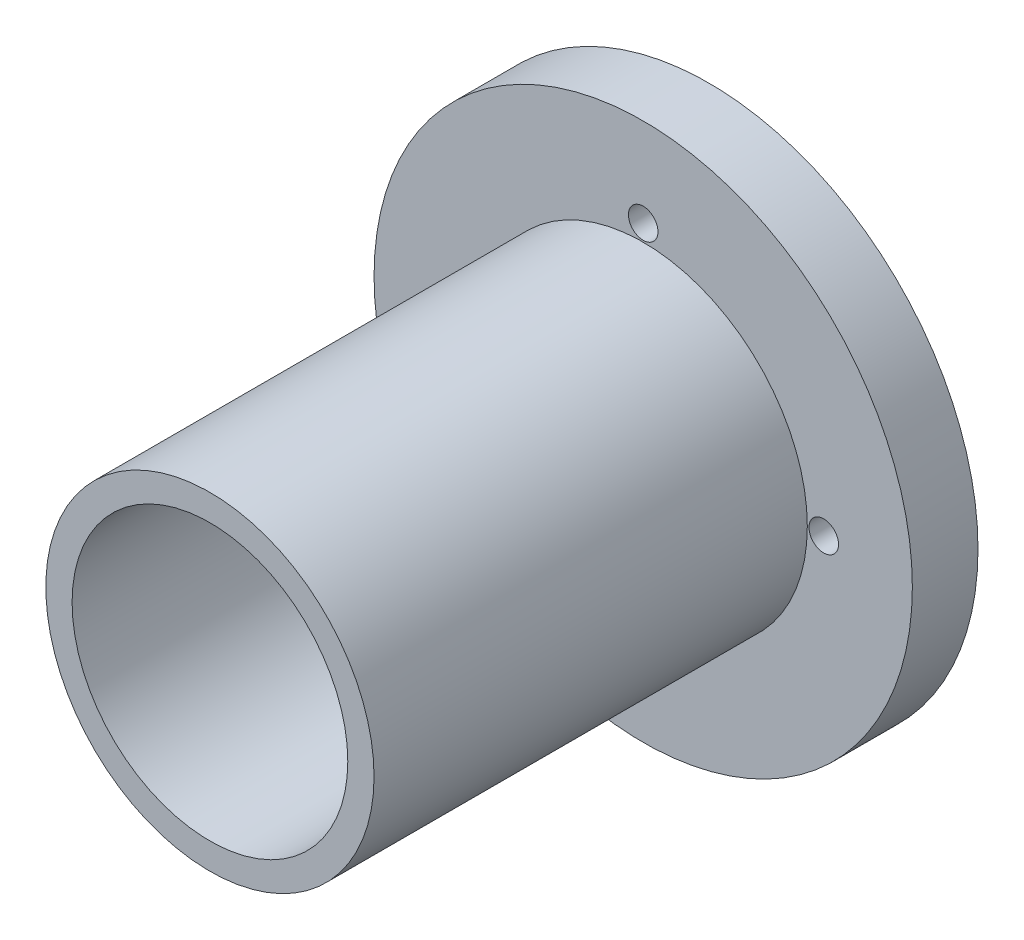
from build123d import *
from build123d.topology import SkipClean

# Parameters (mm, degrees)
SKETCH_1_R                = 25
SKETCH_1_R_2              = 21
EXTRUDE_1_DEPTH           = 66
EXTRUDE_START             = 10
SKETCH_2_R                = 41
SKETCH_2_R_2              = 21
EXTRUDE_2_DEPTH           = 10
HOLE_WIZARD_1_D           = 4.5
HOLE_WIZARD_1_CBORE_D     = 8
HOLE_WIZARD_1_CBORE_DEPTH = 4.6
PATTERN_CIRCULAR_1_COUNT  = 4


with BuildPart() as part:
    # 草图1 → 凸台-拉伸1 (new body)
    with BuildSketch(Plane.XY):
        Circle(SKETCH_1_R)
        Circle(SKETCH_1_R_2, mode=Mode.SUBTRACT)
    extrude(amount=EXTRUDE_1_DEPTH)

    # 草图2 → 凸台-拉伸2 (add)
    with SkipClean():  # the faces are left unmerged after this step: merging them gives an invalid solid
        with BuildSketch(Plane(origin=(0, 0, 0), x_dir=(-1, 0, 0), z_dir=(0, 0, -1)).offset(EXTRUDE_START)):
            Circle(SKETCH_2_R)
            Circle(SKETCH_2_R_2, mode=Mode.SUBTRACT)
        extrude(amount=-EXTRUDE_2_DEPTH)

    # 打孔尺寸(%根据)内六角圆柱头螺钉的类型1 (through all)
    with Locations(Plane(origin=(0, -27.5, -10), x_dir=(-1, 0, 0), z_dir=(0, 0, -1))):
        with Locations((0, 0)):
            hole_wizard_1 = CounterBoreHole(HOLE_WIZARD_1_D / 2, HOLE_WIZARD_1_CBORE_D / 2, HOLE_WIZARD_1_CBORE_DEPTH)

    # 阵列(圆周)1: 打孔尺寸(%根据)内六角圆柱头螺钉的类型1 ×4 about axis
    with SkipClean():  # the faces are left unmerged after this step: merging them gives an invalid solid
        pattern_circular_1_axis = Axis((0, 0, 0), (0, 0, 1))
        for i in range(1, PATTERN_CIRCULAR_1_COUNT):
            add(hole_wizard_1.rotate(pattern_circular_1_axis, i * 360 / PATTERN_CIRCULAR_1_COUNT), mode=Mode.SUBTRACT)


solid = part.part
